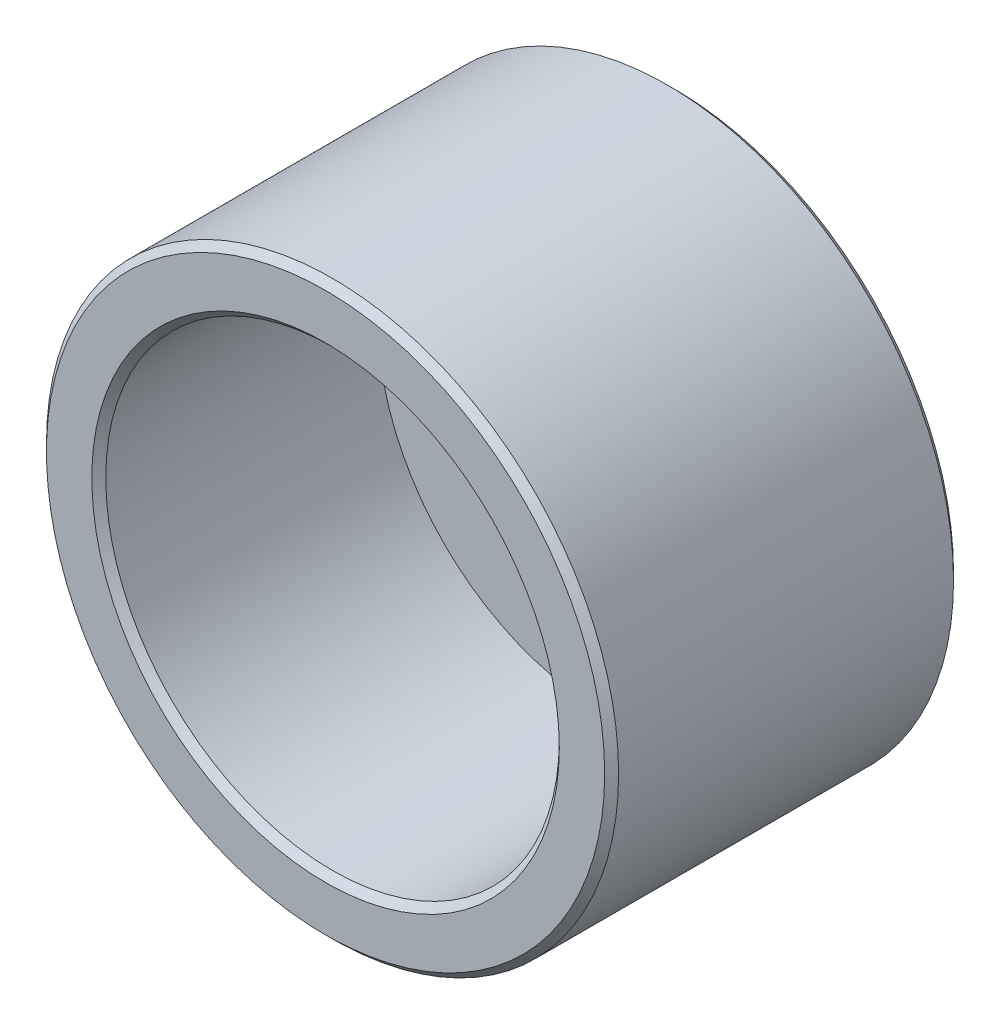
from build123d import *

# Parameters (mm, degrees)
SKETCH1_R           = 20.5
BOSS_EXTRUDE1_DEPTH = 25
CHAMFER1_SIZE       = 0.5
SKETCH5_R           = 16.25
CUT_EXTRUDE1_DEPTH  = 20
CHAMFER2_SIZE       = 0.5
SKETCH6_R           = 10.5
CUT_EXTRUDE2_DEPTH  = 31


with BuildPart() as part:
    # Sketch1 → Boss-Extrude1 (new body)
    with BuildSketch(Plane.XY):
        Circle(SKETCH1_R)
    extrude(amount=BOSS_EXTRUDE1_DEPTH)

    # Chamfer1
    chamfer1_edges = [part.edges().sort_by_distance(p)[0] for p in [
        (-20.5, 0, 0),
        (-20.5, 0, 25),
    ]]
    chamfer(chamfer1_edges, length=CHAMFER1_SIZE)

    # Sketch5 → Cut-Extrude1 (cut)
    with BuildSketch(Plane.XY.offset(25)):
        Circle(SKETCH5_R)
    extrude(amount=-CUT_EXTRUDE1_DEPTH, mode=Mode.SUBTRACT)

    # Chamfer2
    chamfer2_edges = [part.edges().sort_by_distance(p)[0] for p in [
        (-16.25, 0, 25),
    ]]
    chamfer(chamfer2_edges, length=CHAMFER2_SIZE)

    # Sketch6 → Cut-Extrude2 (cut)
    with BuildSketch(Plane(origin=(0, 0, 0), x_dir=(-1, 0, 0), z_dir=(0, 0, -1))):
        Circle(SKETCH6_R)
    extrude(amount=-CUT_EXTRUDE2_DEPTH, mode=Mode.SUBTRACT)


solid = part.part
